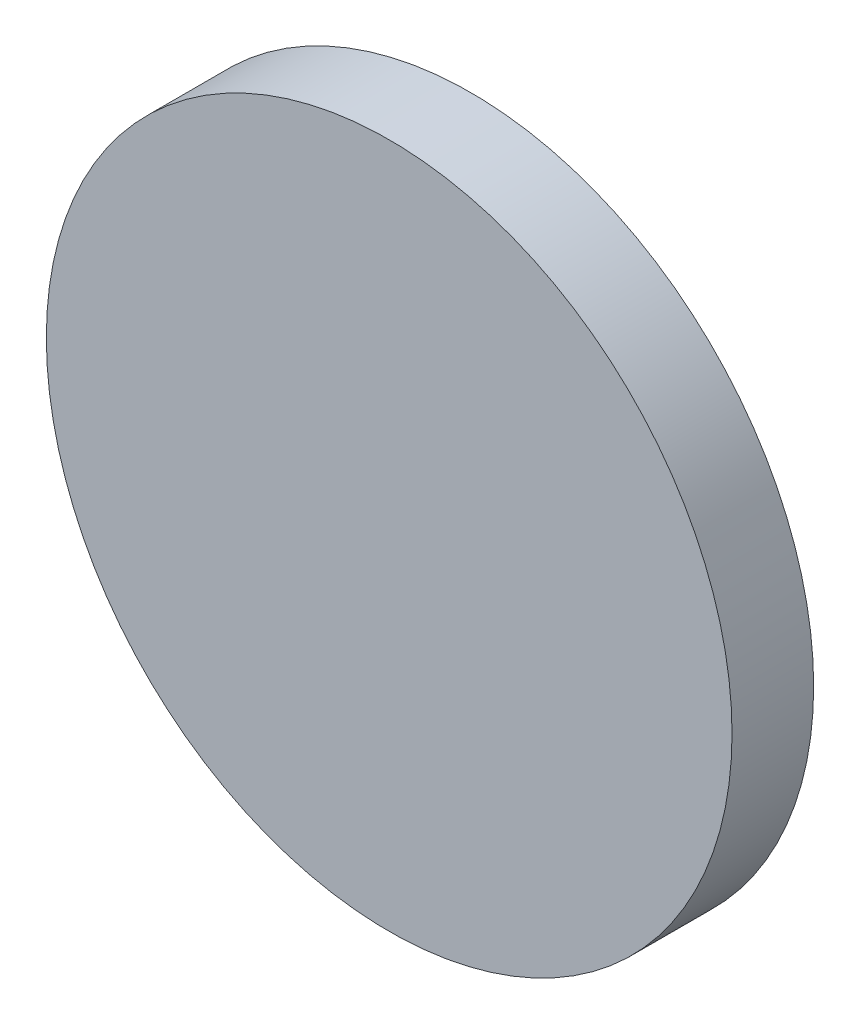
from build123d import *

# Parameters (mm, degrees)
SKETCH_1_R      = 42
EXTRUDE_1_DEPTH = 5


with BuildPart() as part:
    # 草图1 → 凸台-拉伸1 (new, symmetric)
    with BuildSketch(Plane.XY):
        Circle(SKETCH_1_R)
    extrude(amount=EXTRUDE_1_DEPTH, both=True)


solid = part.part
